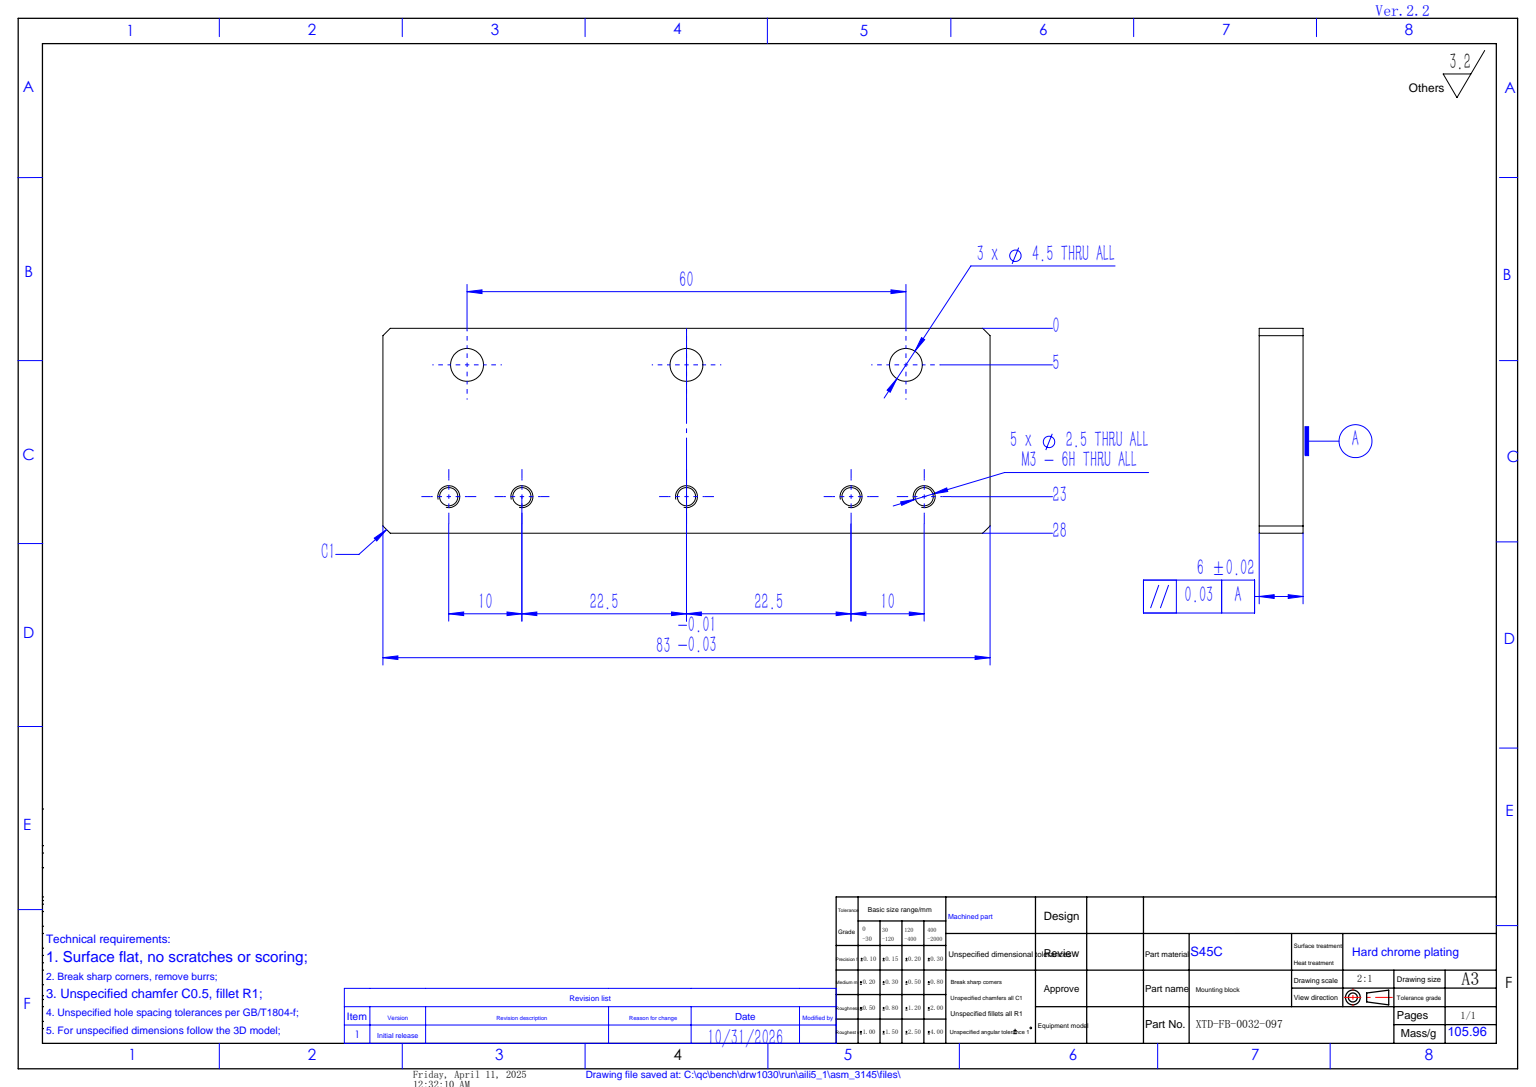
SolidWorks part; units mm, degrees
material "S45C"
ref_plane "前视基准面" through (0, 0, 0) normal (0, 0, 1) x (1, 0, 0)
ref_plane "上视基准面" through (0, 0, 0) normal (0, 1, 0) x (1, 0, 0)
ref_plane "右视基准面" through (0, 0, 0) normal (1, 0, 0) x (0, 0, -1)
sketch "草图1" plane through (0, 0, 0) normal (0, 0, 1) x (1, 0, 0)
  line L1 (-41.5, 14) -> (41.5, 14)
  line L2 (-41.5, 14) -> (-41.5, -14)
  line L3 (-41.5, -14) -> (41.5, -14)
  line L4 (41.5, 14) -> (41.5, -14)
  line L5 (-41.5, 14) -> (41.5, -14) construction
  line L6 (-41.5, -14) -> (41.5, 14) construction
  point P0 (0, 0)
  dimension "D1" = 83
  dimension "D2" = 28
extrude "凸台-拉伸1" add sketch "草图1" along normal blind 6
hole_wizard "M4 间隙孔1" positions "草图2" profile "草图3" hole size "M4" standard "ISO" end condition through all
sketch "草图2" plane through (0, 0, 6) normal (0, 0, 1) x (1, 0, 0)
  line L0 (0, 0.6056) -> (0, 23.0141) construction
  line L1 (41.5, 14) -> (-41.5, 14) construction
  point P0 (-30, 9)
  point P7 (0, 9)
  point P10 (30, 9)
  dimension "D1" = 60
  dimension "D2" = 5
sketch "草图3" plane through (-30, 9, 6) normal (1, 0, 0) x (0, -1, 0)
  line L0 (0, 0) -> (0, 6)
  line L1 (0, 6) -> (2.25, 6)
  line L2 (2.25, 6) -> (2.25, 0)
  line L5 (2.25, 0) -> (0, 0)
  line L11 (0, -6.35) -> (0, 107.95) construction
  dimension "通孔孔直径" = 4.5
  dimension "通孔孔深度" = 6
hole_wizard "M3 螺纹孔1" positions "草图4" profile "草图5" tap size "M3" standard "ISO" end condition through all
sketch "草图4" plane through (0, 0, 6) normal (0, 0, 1) x (1, 0, 0)
  line L0 (0, 0) -> (0, 22.9601) construction
  line L1 (-41.5, -14) -> (41.5, -14) construction
  point P0 (-32.5, -9)
  point P3 (0, -9)
  point P5 (32.5, -9)
  point P11 (22.5, -9)
  point P14 (-22.5, -9)
  dimension "D1" = 65
  dimension "D2" = 45
  dimension "D3" = 5
sketch "草图5" plane through (-32.5, -9, 6) normal (1, 0, 0) x (0, -1, 0)
  line L0 (0, 0) -> (0, 6)
  line L1 (0, 6) -> (1.25, 6)
  line L2 (1.25, 6) -> (1.25, 0)
  line L5 (1.25, 0) -> (0, 0)
  line L11 (0, -6.35) -> (0, 107.95) construction
  dimension "通孔螺纹孔钻头直径" = 2.5
  dimension "通孔螺纹孔钻头深度" = 6
cosmetic thread "孔螺蚊线1" parameters "D2"=3
cosmetic thread "孔螺蚊线2" parameters "D2"=3
cosmetic thread "孔螺蚊线3" parameters "D2"=3
cosmetic thread "孔螺蚊线4" parameters "D2"=3
cosmetic thread "孔螺蚊线5" parameters "D2"=3
chamfer "倒角1" distance 1 angle 45 4 edges at (41.5, 14, 3) (41.5, -14, 3) (-41.5, -14, 3) (-41.5, 14, 3)
